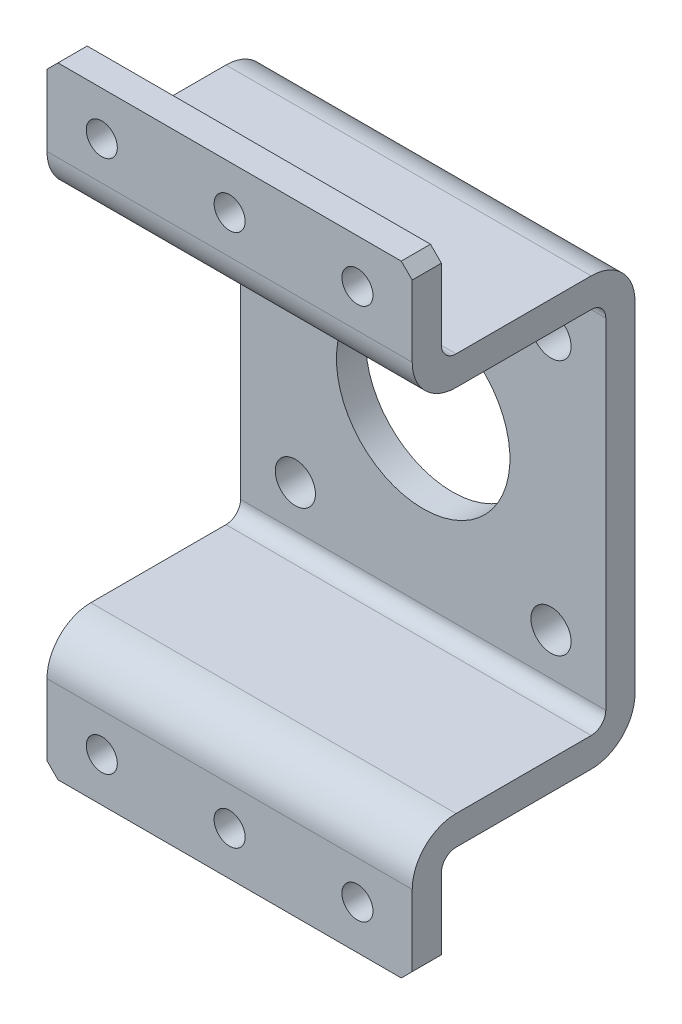
from build123d import *

# Parameters (mm, degrees)
EXTRUDE_1_DEPTH         = 50
SKETCH_3_R              = 23.75
CUT_EXTRUDE_1_DEPTH     = 116.956888541
HOLE_WIZARD_11_0_11_1_D = 11
HOLE_WIZARD_8_5_8_5_1_D = 8.5
CHAMFER_1_SIZE          = 3
FILLET_1_R              = 4
FILLET_2_R              = 12


with BuildPart() as part:
    # 草图1 → 凸台-拉伸1 (new, symmetric)
    with BuildSketch(Plane(origin=(0, 0, 0), x_dir=(0, 0, -1), z_dir=(1, 0, 0))):
        Polygon((-61, 85), (-61, 50.5), (-8, 50.5), (-8, -50.5), (-61, -50.5), (-61, -85), (-53, -85), (-53, -58.5), (0, -58.5), (0, 58.5), (-53, 58.5), (-53, 85), align=None)
    extrude(amount=EXTRUDE_1_DEPTH, both=True)

    # 草图3 → 切除-拉伸1 (cut, through all)
    with BuildSketch(Plane(origin=(0, 0, 0), x_dir=(-1, 0, 0), z_dir=(0, 0, -1))):
        with Locations(Location((0, 0, 0), (0, 0, 90))):
            Circle(SKETCH_3_R)
    extrude(amount=-CUT_EXTRUDE_1_DEPTH, mode=Mode.SUBTRACT)

    # Ø11.0 (11) 直径孔1 (through all)
    with Locations(Plane(origin=(0, 0, 0), x_dir=(-1, 0, 0), z_dir=(0, 0, -1))):
        with Locations((0, 0), (35, -35), (-35, 35), (-35, -35), (35, 35)):
            Hole(HOLE_WIZARD_11_0_11_1_D / 2)

    # Ø8.5 (8.5) 直径孔1 (through all)
    with Locations(Plane(origin=(0, 0, 53), x_dir=(-1, 0, 0), z_dir=(0, 0, -1))):
        with Locations((-35, -73), (0, -73), (35, -73), (35, 73), (0, 73), (-35, 73)):
            Hole(HOLE_WIZARD_8_5_8_5_1_D / 2)

    # 倒角1
    chamfer_1_edges = [part.edges().sort_by_distance(p)[0] for p in [
        (-50, -85, 57),
        (-50, 85, 57),
        (50, -85, 57),
        (50, 85, 57),
    ]]
    chamfer(chamfer_1_edges, length=CHAMFER_1_SIZE)

    # 圆角1
    fillet_1_edges = [part.edges().sort_by_distance(p)[0] for p in [
        (0, 58.5, 53),
        (0, -58.5, 53),
        (0, -50.5, 8),
        (0, 50.5, 8),
    ]]
    fillet(fillet_1_edges, radius=FILLET_1_R)

    # 圆角2
    fillet_2_edges = [part.edges().sort_by_distance(p)[0] for p in [
        (0, 58.5, 0),
        (0, -58.5, 0),
        (0, -50.5, 61),
        (0, 50.5, 61),
    ]]
    fillet(fillet_2_edges, radius=FILLET_2_R)


solid = part.part
